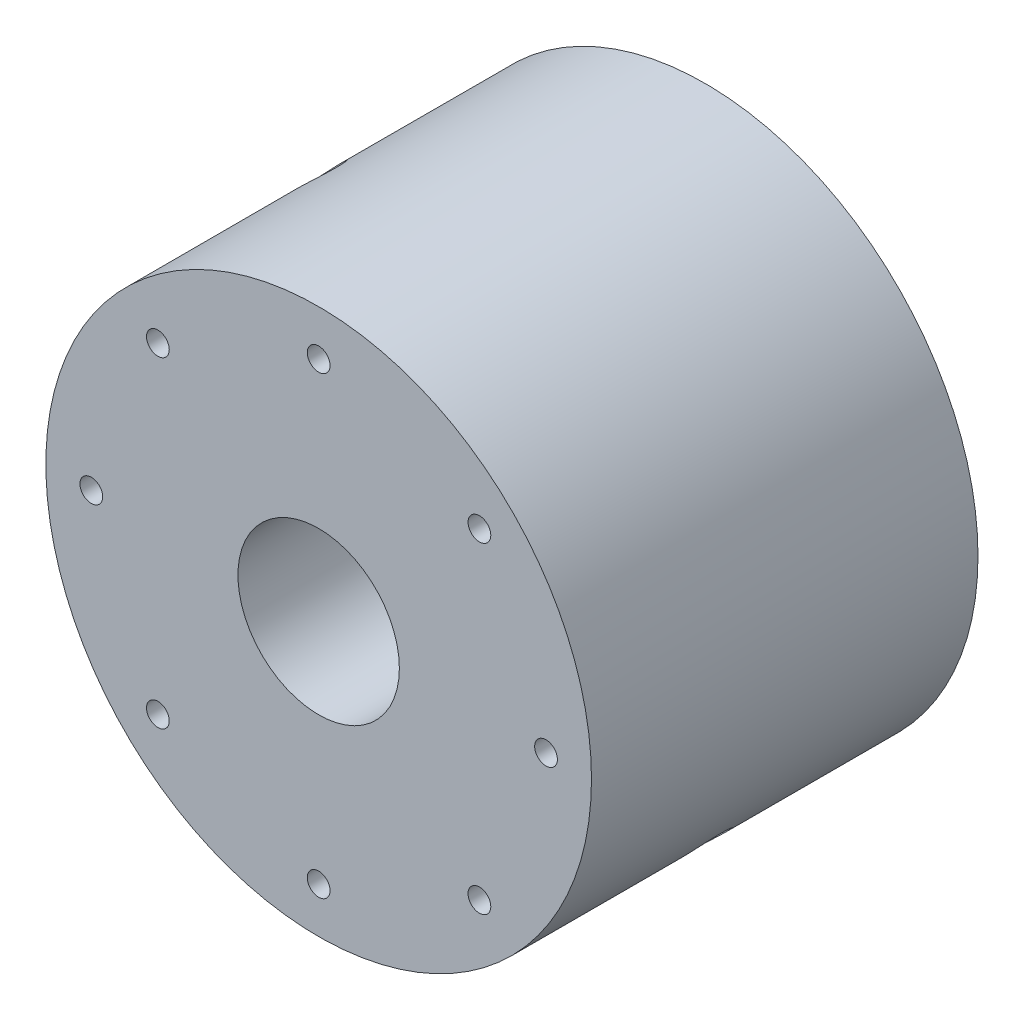
from build123d import *

# Parameters (mm, degrees)
SKETCH_1_R               = 60
SKETCH_1_R_2             = 17.75
EXTRUDE_1_DEPTH          = 42.5
PATTERN_CIRCULAR_1_COUNT = 8
PATTERN_CIRCULAR_2_COUNT = 4
SKETCH_6_R               = 5
CUT_EXTRUDE_1_DEPTH      = 90


with BuildPart() as part:
    # 草图1 → 凸台-拉伸1 (new, symmetric)
    with BuildSketch(Plane.XY):
        Circle(SKETCH_1_R)
        Circle(SKETCH_1_R_2, mode=Mode.SUBTRACT)
    extrude(amount=EXTRUDE_1_DEPTH, both=True)

    # 草图3 → M6x1.0 螺纹孔1 (revolve, cut)
    with BuildSketch(Plane(origin=(0, 50, 42.5), x_dir=(0, -1, 0), z_dir=(1, 0, 0))):
        Polygon((0, 0), (0, 16.502151548), (2.5, 15), (2.5, 0), align=None)
    m6x1_0_1 = revolve(axis=Axis((0, 50, 48.85), (0, 0, -1)), mode=Mode.SUBTRACT)

    # 阵列(圆周)1: M6x1.0 螺纹孔1 ×8 about axis
    pattern_circular_1_axis = Axis((0, 0, 0), (0, 0, 1))
    for i in range(1, PATTERN_CIRCULAR_1_COUNT):
        add(m6x1_0_1.rotate(pattern_circular_1_axis, i * 360 / PATTERN_CIRCULAR_1_COUNT), mode=Mode.SUBTRACT)

    # 草图5 → M4x0.7 螺纹孔1 (revolve, cut)
    with BuildSketch(Plane(origin=(-36, 0, -42.5), x_dir=(0, 1, 0), z_dir=(1, 0, 0))):
        Polygon((0, 0), (0, 11.091420021), (1.65, 10.1), (1.65, 0), align=None)
    m4x0_7_1 = revolve(axis=Axis((-36, 0, -48.85), (0, 0, 1)), mode=Mode.SUBTRACT)

    # 阵列(圆周)2: M4x0.7 螺纹孔1 ×4 about axis
    pattern_circular_2_axis = Axis((0, 0, 0), (0, 0, 1))
    for i in range(1, PATTERN_CIRCULAR_2_COUNT):
        add(m4x0_7_1.rotate(pattern_circular_2_axis, i * 360 / PATTERN_CIRCULAR_2_COUNT), mode=Mode.SUBTRACT)

    # 草图6 → 切除-拉伸1 (cut, symmetric)
    with BuildSketch(Plane(origin=(0, 0, 0), x_dir=(-0.7071067811865438, -0.7071067811865512, 0), z_dir=(0.7071067811865512, -0.7071067811865438, 0))):
        with Locations(Location((0, 0, 0), (0, 0, 180))):
            Circle(SKETCH_6_R)
    extrude(amount=CUT_EXTRUDE_1_DEPTH, both=True, mode=Mode.SUBTRACT)


solid = part.part
